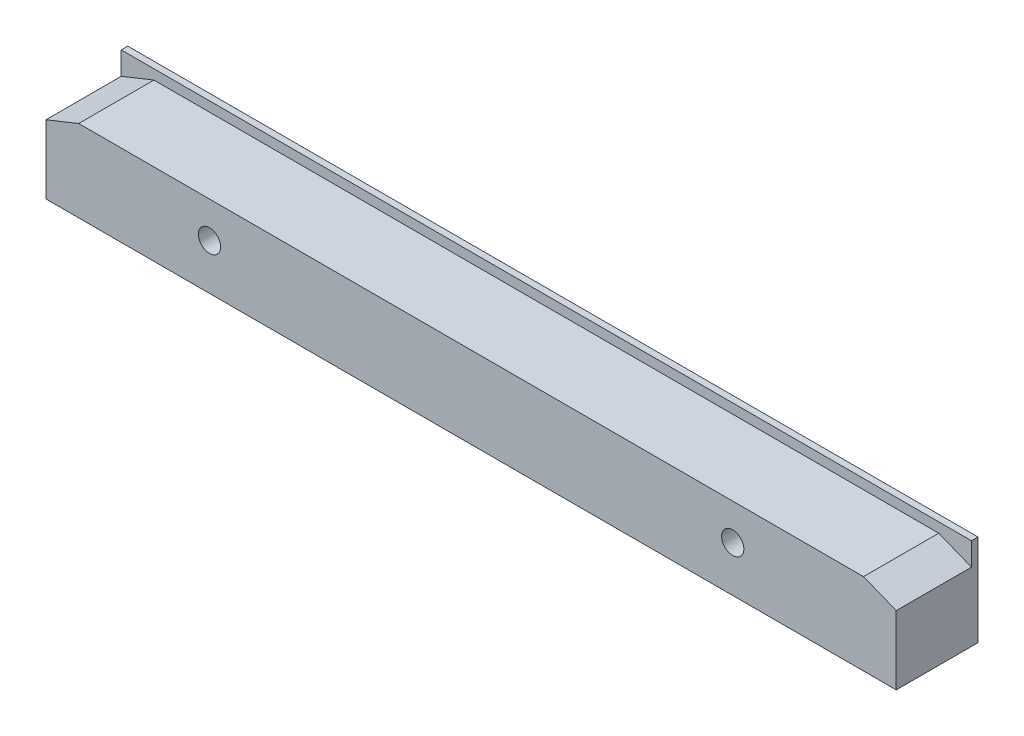
from build123d import *

# Parameters (mm, degrees)
SKETCH_1_W                = 130
SKETCH_1_H                = 14
EXTRUDE_1_DEPTH           = 12.5
SKETCH_2_W                = 11.5
SKETCH_2_H                = 1.5
CUT_EXTRUDE_1_DEPTH       = 131.787040642
CHAMFER_3_SIZE            = 2
CHAMFER_3_SIZE2           = 5
CHAMFER_4_SIZE            = 5
CHAMFER_4_SIZE2           = 2
HOLE_WIZARD_1_D           = 3.4
HOLE_WIZARD_1_CBORE_D     = 6
HOLE_WIZARD_1_CBORE_DEPTH = 3.4


with BuildPart() as part:
    # 草图1 → 凸台-拉伸1 (new body)
    with BuildSketch(Plane.XY):
        Rectangle(SKETCH_1_W, SKETCH_1_H)
    extrude(amount=EXTRUDE_1_DEPTH)

    # 草图2 → 切除-拉伸1 (cut, through all)
    with BuildSketch(Plane(origin=(65, 0, 0), x_dir=(0, 0, -1), z_dir=(1, 0, 0))):
        with Locations((-6.75, 6.25)):
            Rectangle(SKETCH_2_W, SKETCH_2_H)
    extrude(amount=-CUT_EXTRUDE_1_DEPTH, mode=Mode.SUBTRACT)

    # 倒角3
    chamfer_3_edges = [part.edges().sort_by_distance(p)[0] for p in [
        (65, 5.5, 6.75),
    ]]
    chamfer_3_side = [part.faces().sort_by_distance(p)[0] for p in [
        (65, -0.683438986, 6.195324881),
    ]]
    chamfer(chamfer_3_edges, length=CHAMFER_3_SIZE, length2=CHAMFER_3_SIZE2, reference=chamfer_3_side[0])

    # 倒角4
    chamfer_4_edges = [part.edges().sort_by_distance(p)[0] for p in [
        (-65, 5.5, 6.75),
    ]]
    chamfer_4_side = [part.faces().sort_by_distance(p)[0] for p in [
        (-2.5, 5.5, 6.75),
    ]]
    chamfer(chamfer_4_edges, length=CHAMFER_4_SIZE, length2=CHAMFER_4_SIZE2, reference=chamfer_4_side[0])

    # 打孔尺寸根据内六角圆柱头螺钉的类型1 (through all)
    with Locations(Plane(origin=(0, 0, 0), x_dir=(-1, 0, 0), z_dir=(0, 0, -1))):
        with Locations((-40, 0), (40, 0)):
            CounterBoreHole(HOLE_WIZARD_1_D / 2, HOLE_WIZARD_1_CBORE_D / 2, HOLE_WIZARD_1_CBORE_DEPTH)


solid = part.part
